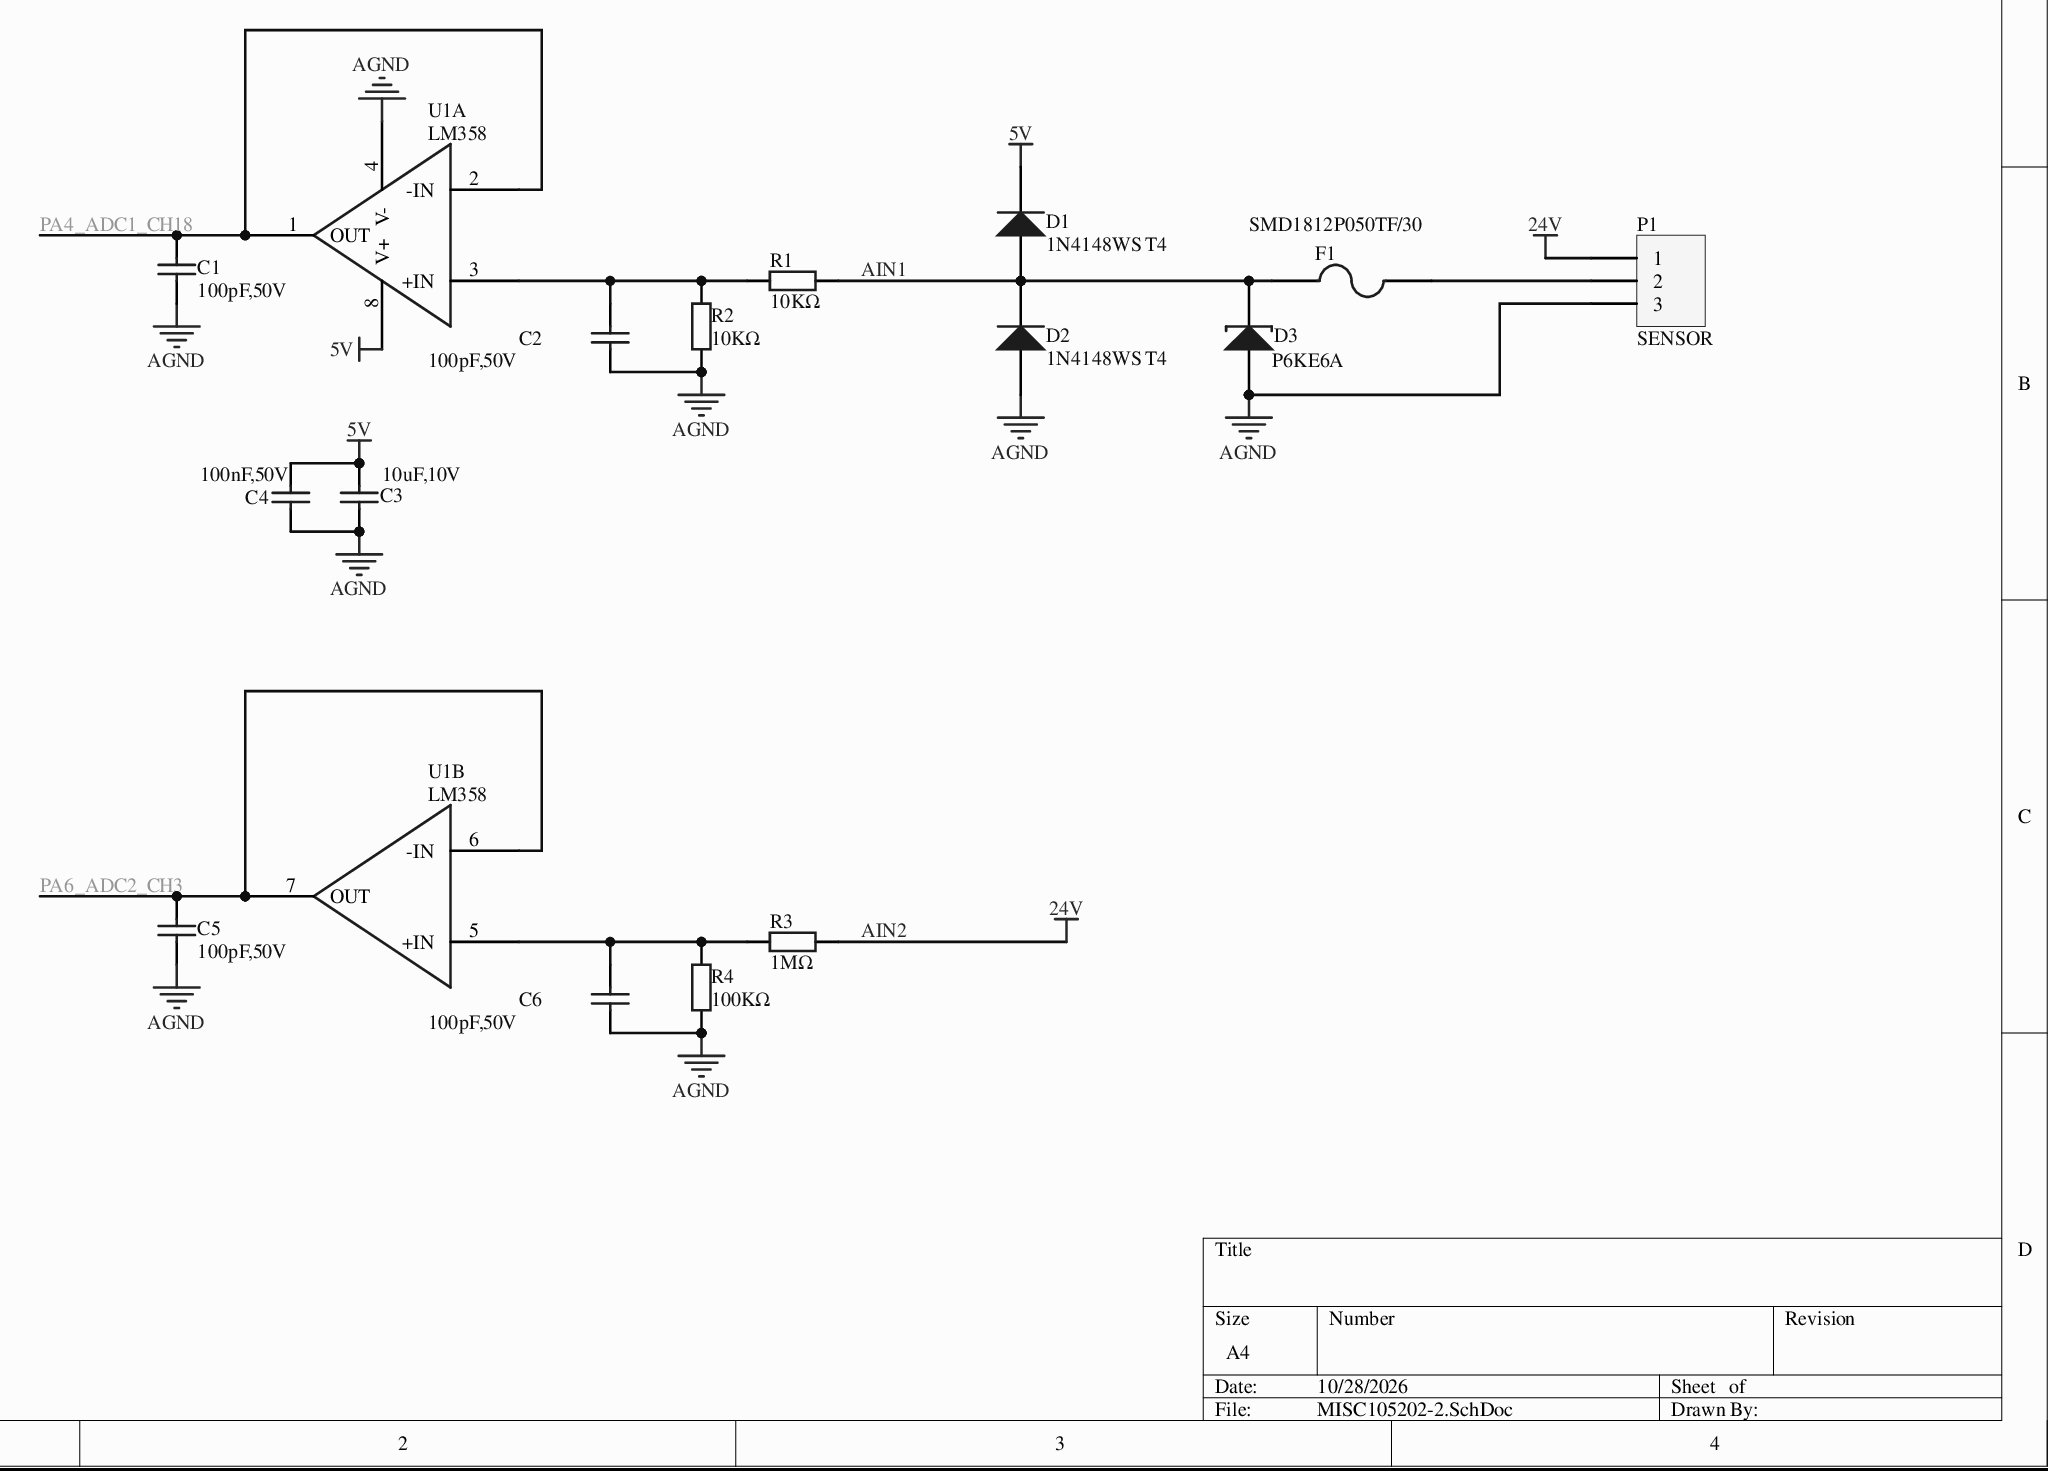
[diagram p0: MISC105202-2.SchDoc]
# Altium project MISC105202-19.PrjPCB (part 1 of 3)
7 sheets, 181 parts. Net scope: global (net labels, ports and power ports of the same name join across sheets).
Board file: MISC105202-15.PcbDoc
Sheets:
  MISC105202-2.SchDoc
  MISC105202-4.SchDoc
  PCBE105202.SchDoc
  MISC105202-9.SchDoc
  MISC105202-21.SchDoc
  MISC105202-13.SchDoc
  MISC105202-24.SchDoc

## Sheet MISC105202-2.SchDoc
size A4

### Parts
C1  100pF,50V  [0603_C]
C2  100pF,50V  [0603_C]
C3  10uF,10V  [0603_C]
C4  100nF,50V  [0603_C]
C5  100pF,50V  [0603_C]
C6  100pF,50V  [0603_C]
D1  1N4148WS T4  [SOD-323]
D2  1N4148WS T4  [SOD-323]
D3  P6KE6A  [P6KESMD]
F1  SMD1812P050TF/30  [1812]
P1  SENSOR  [508*3]
R1  10KΩ  [0603_R]
R2  10KΩ  [0603_R]
R3  1MΩ  [0603_R]
R4  100KΩ  [0603_R]
U1  LM358  [SO-8]  (parts A,B of 2)

### Nets
5V: C3.2 C4.2 D1.2(K) U1.8(V+)
AGND: C1.1 C2.1 C3.1 C4.1 C5.1 C6.1 D2.1(A) D3.1(A) P1.3 R2.1 R4.1 U1.4(V-)
AIN2: P1.1 R3.2  [also labelled 24V]
AIN1: D1.1(A) D2.2(K) D3.2(K) F1.2 R1.2
PA4_ADC1_CH18: C1.2 U1.1(OUT) U1.2(-IN)
PA6_ADC2_CH3: C5.2 U1.6(-IN) U1.7(OUT)
NetC2_2: C2.2 R1.1 R2.2 U1.3(+IN)
NetC6_2: C6.2 R3.1 R4.2 U1.5(+IN)
NetF1_1: F1.1 P1.2

### Library data of the parts
C1 C2 C5 C6 = 0603 100pF (101) 5% 50V: 贴片电容; ComponentLink1Description: supplier link; Package: 0603; Supplier: LC; SuppliersPartNumber: C14858
C3 = 0603 10uF (106) 10% 10V: 贴片电容; ComponentLink1Description: supplier link; Package: 0603; Supplier: LC; SuppliersPartNumber: C19702
C4 = 0603 100nF (104) 10% 50V: 贴片电容; ComponentLink1Description: supplier link; Package: 0603; Supplier: LC; SuppliersPartNumber: C14663
D1 D2 = SOD-323 1N4148WS T4: 二极管; ComponentLink1Description: supplier link; Package: SOD-323; Supplier: LC; SuppliersPartNumber: C2128
D3 = D Tunnel2: Tunnel Diode - Dependent Source Model; Published: 15-Apr-2002; LatestRevisionDate: 17-Jul-2002; LatestRevisionNote: Re-released for DXP Platform.; PackageReference: DIODE-0.4; Publisher: Altium Limited
F1 = Fuse 2: Fuse; Published: 8-Jun-2000; LatestRevisionDate: 17-Jul-2002; LatestRevisionNote: Re-released for DXP Platform.; PackageReference: PIN-W2/E2.8; Publisher: Altium Limited
P1 = Header 3: Header, 3-Pin; LatestRevisionDate: 17-Jul-2002; LatestRevisionNote: Re-released for DXP Platform.; Publisher: Altium Limited
R1-R4 = 0603 10KΩ (1002) 1%: 贴片电阻; ComponentLink1Description: supplier link; Package: 0603; Supplier: LC; SuppliersPartNumber: C25804
U1 = OPA2335

## Sheet MISC105202-4.SchDoc
size A4
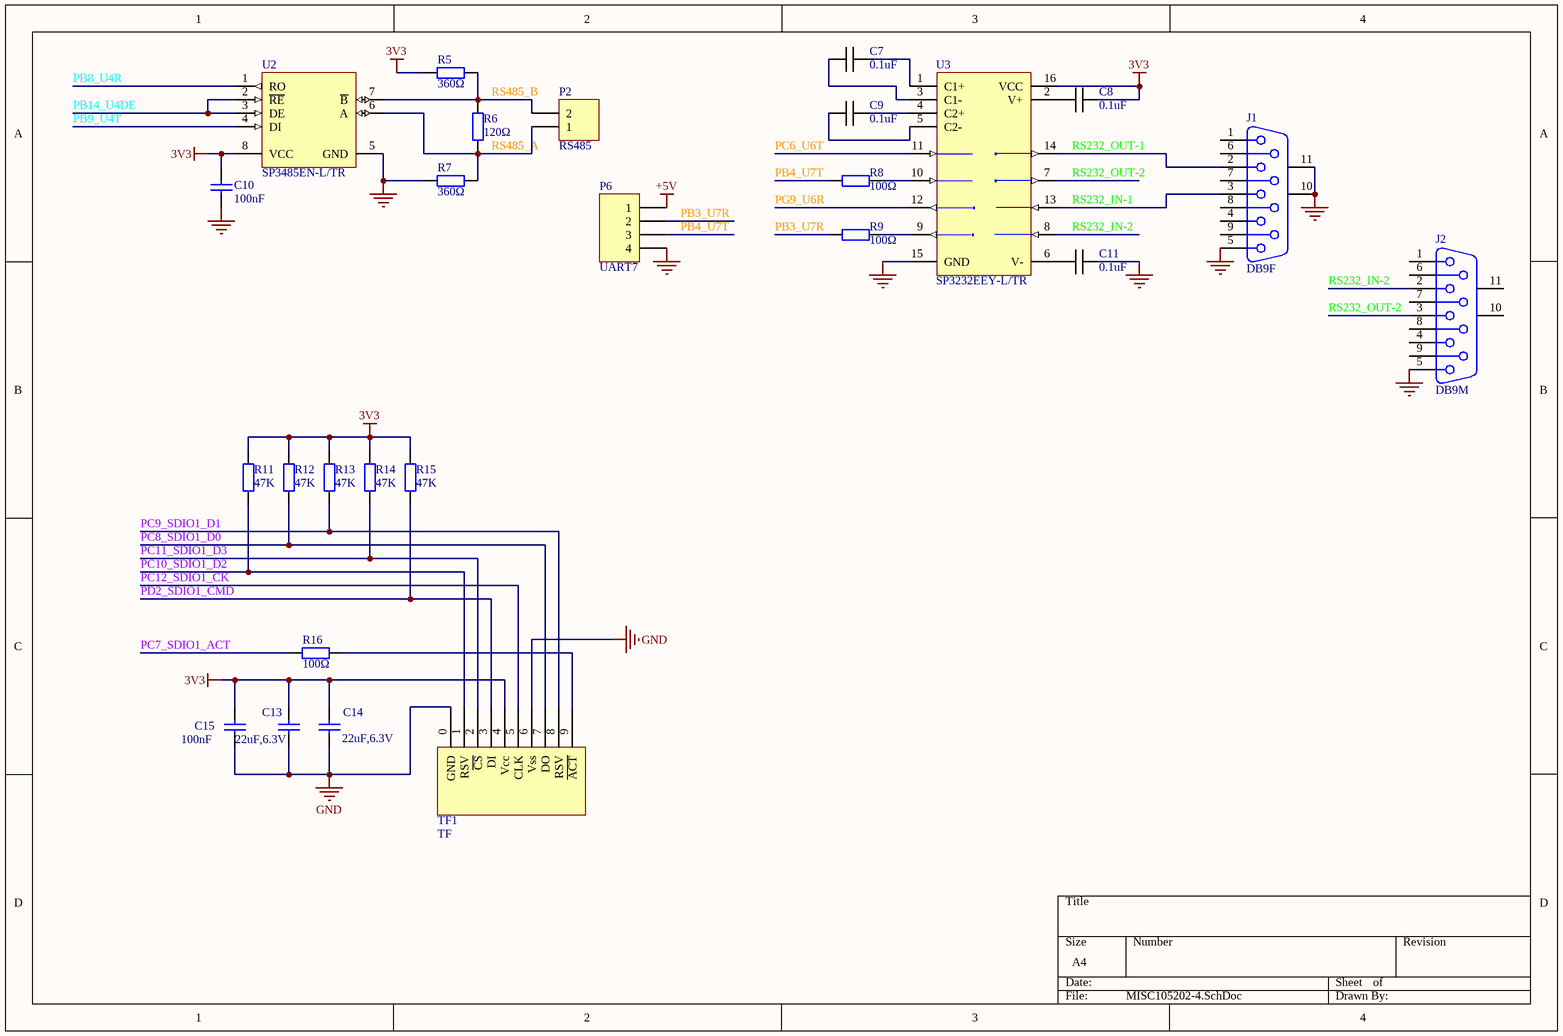
[diagram p1: MISC105202-4.SchDoc]

### Parts
C7  0.1uF  [0603_C]
C8  0.1uF  [0603_C]
C9  0.1uF  [0603_C]
C10  100nF  [0603_C]
C11  0.1uF  [0603_C]
C13  22uF,6.3V  [0603_C]
C14  22uF,6.3V  [0603_C]
C15  100nF  [0402_C]
J1  DB9F  [DB9RA/F]
J2  DB9M  [DB9RA/M]
P2  RS485  [508*2B]
P6  UART7  [HDR1X4]
R5  360Ω  [0603_R]
R6  120Ω  [0603_R]
R7  360Ω  [0603_R]
R8  100Ω  [0603_R]
R9  100Ω  [0603_R]
R11  47K  [0402_R]
R12  47K  [0402_R]
R13  47K  [0402_R]
R14  47K  [0402_R]
R15  47K  [0402_R]
R16  100Ω  [0402_R]
TF1  TF  [MICROSD]
U2  SP3485EN-L/TR  [SOIC-8_150mil]
U3  SP3232EEY-L/TR  [TSSOP-16]

### Nets
3V3: C8.1 C10.2 C13.2 C14.2 C15.2 R5.1 R11.2 R12.2 R13.2 R14.2 R15.2 TF1.4(Vcc) U2.8(VCC) U3.16(VCC)
+5V: P6.1
GND: C10.1 C11.1 C13.1 C14.1 C15.1 J1.5 J1.10(MH1) J1.11(MH2) J2.5 P6.4 R7.1 TF1.0(GND) TF1.6(Vss) U2.5(GND) U3.15(GND)
PB3_U7R: P6.2 R9.1  [project net PB3_SDIO2_D2]
PB4_U7T: P6.3 R8.1  [project net PB4_SDIO2_D3]
PB8_U4R: U2.1(RO)  [project net PB8_SDIO1_CKIN]
PB9_U4T: U2.4(DI)  [project net PB9_SDIO1_CDIR]
PB14_U4DE: U2.2(~{RE}) U2.3(DE)  [project net PB14_SDIO2_D0]
PC6_U6T: U3.11(T1IN)  [project net PC6_SDIO1_D0DIR]
PC7_SDIO1_ACT: R16.1
PC8_SDIO1_D0: R12.1 TF1.7(DO)
PC9_SDIO1_D1: R13.1 TF1.8(RSV)
PC10_SDIO1_D2: R11.1 TF1.1(RSV)
PC11_SDIO1_D3: R14.1 TF1.2(~{CS})
PC12_SDIO1_CK: TF1.5(CLK)
PD2_SDIO1_CMD: R15.1 TF1.3(DI)
PG9_U6R: U3.12(R1OUT)  [project net PG9_QSPI_BK2_IO2]
RS232_IN-1: J1.3 U3.13(R1IN)
RS232_IN-2: J2.2 U3.8(R2IN)
RS232_OUT-1: J1.2 U3.14(T1OUT)
RS232_OUT-2: J2.3 U3.7(T2OUT)
RS485_A: P2.1 R6.2 R7.2 U2.6(A)
RS485_B: P2.2 R5.2 R6.1 U2.7(~{B})
NetC7_1: C7.1 U3.1(C1+)
NetC7_2: C7.2 U3.3(C1-)
NetC8_2: C8.2 U3.2(V+)
NetC9_1: C9.1 U3.4(C2+)
NetC9_2: C9.2 U3.5(C2-)
NetC11_2: C11.2 U3.6(V-)
NetR8_2: R8.2 U3.10(T2IN)
NetR9_2: R9.2 U3.9(R2OUT)
NetR16_2: R16.2 TF1.9(~{ACT})

Not connected (* = marked no-connect by the designer): J1 1 4 6 7 8 9; J2 1 4 6 7 8 9 10(MH1) 11(MH2)

### Library data of the parts
C7-C9 C11 = CAP
C10 = 0603 100nF (104) 10% 50V: 贴片电容; ComponentLink1Description: supplier link; Package: 0603; Supplier: LC; SuppliersPartNumber: C14663
C13 C14 = 0603 22uF (226) 20% 6.3V: 贴片电容; ComponentLink1Description: supplier link; Package: 0603; Supplier: LC; SuppliersPartNumber: C59461
C15 = 0402 100nF (104) 10% 16V: 贴片电容; ComponentLink1Description: supplier link; Package: 0402; Supplier: LC; SuppliersPartNumber: C1525
J1 J2 = D Connector 9: Receptacle Assembly, 9 Position, Right Angle; PackageDocument: O; Positions: 9; Published: 15-Jun-2001; LatestRevisionDate: 17-Jul-2002; LatestRevisionNote: Re-released for DXP Platform.; DatasheetDocument: 1-Sep-1999; PackageReference: 788750; Orientation: Right Angle; Gender: Receptacle; Publisher: Altium Limited
P2 = Header 2: Header, 2-Pin; LatestRevisionDate: 17-Jul-2002; LatestRevisionNote: Re-released for DXP Platform.; Publisher: Altium Limited
P6 = Header 4: Header, 4-Pin; LatestRevisionDate: 17-Jul-2002; LatestRevisionNote: Re-released for DXP Platform.; Publisher: Altium Limited
R5 R7 = 0603 360Ω (3600) 1%: 贴片电阻; ComponentLink1Description: supplier link; Package: 0603; Supplier: LC; SuppliersPartNumber: C25194
R6 = 0603 120Ω (1200) 1%: 贴片电阻; ComponentLink1Description: supplier link; Package: 0603; Supplier: LC; SuppliersPartNumber: C22787
R8 R9 = 0603 100Ω (1000) 1%: 贴片电阻; ComponentLink1Description: supplier link; Package: 0603; Supplier: LC; SuppliersPartNumber: C22775
R11-R15 = 0402 47KΩ (4702) 1%: 贴片电阻; ComponentLink1Description: supplier link; Package: 0402; Supplier: LC; SuppliersPartNumber: C25792
R16 = 0402 100Ω (1000) 1%: 贴片电阻; ComponentLink1Description: supplier link; Package: 0402; Supplier: LC; SuppliersPartNumber: C25076
U2 = SP3485EN-L/TR_[C8963]: RS-485/RS-422; ComponentLink1Description: supplier link; Package: SOIC-8; Supplier: LC; SuppliersPartNumber: C8963
U3 = SP3232EEY-L/TR: RS232; ComponentLink1Description: supplier link; Package: TSSOP-16; Supplier: LC; SuppliersPartNumber: C13482

## Sheet PCBE105202.SchDoc
size A3; SheetNumber: 12; SheetTotal: 14
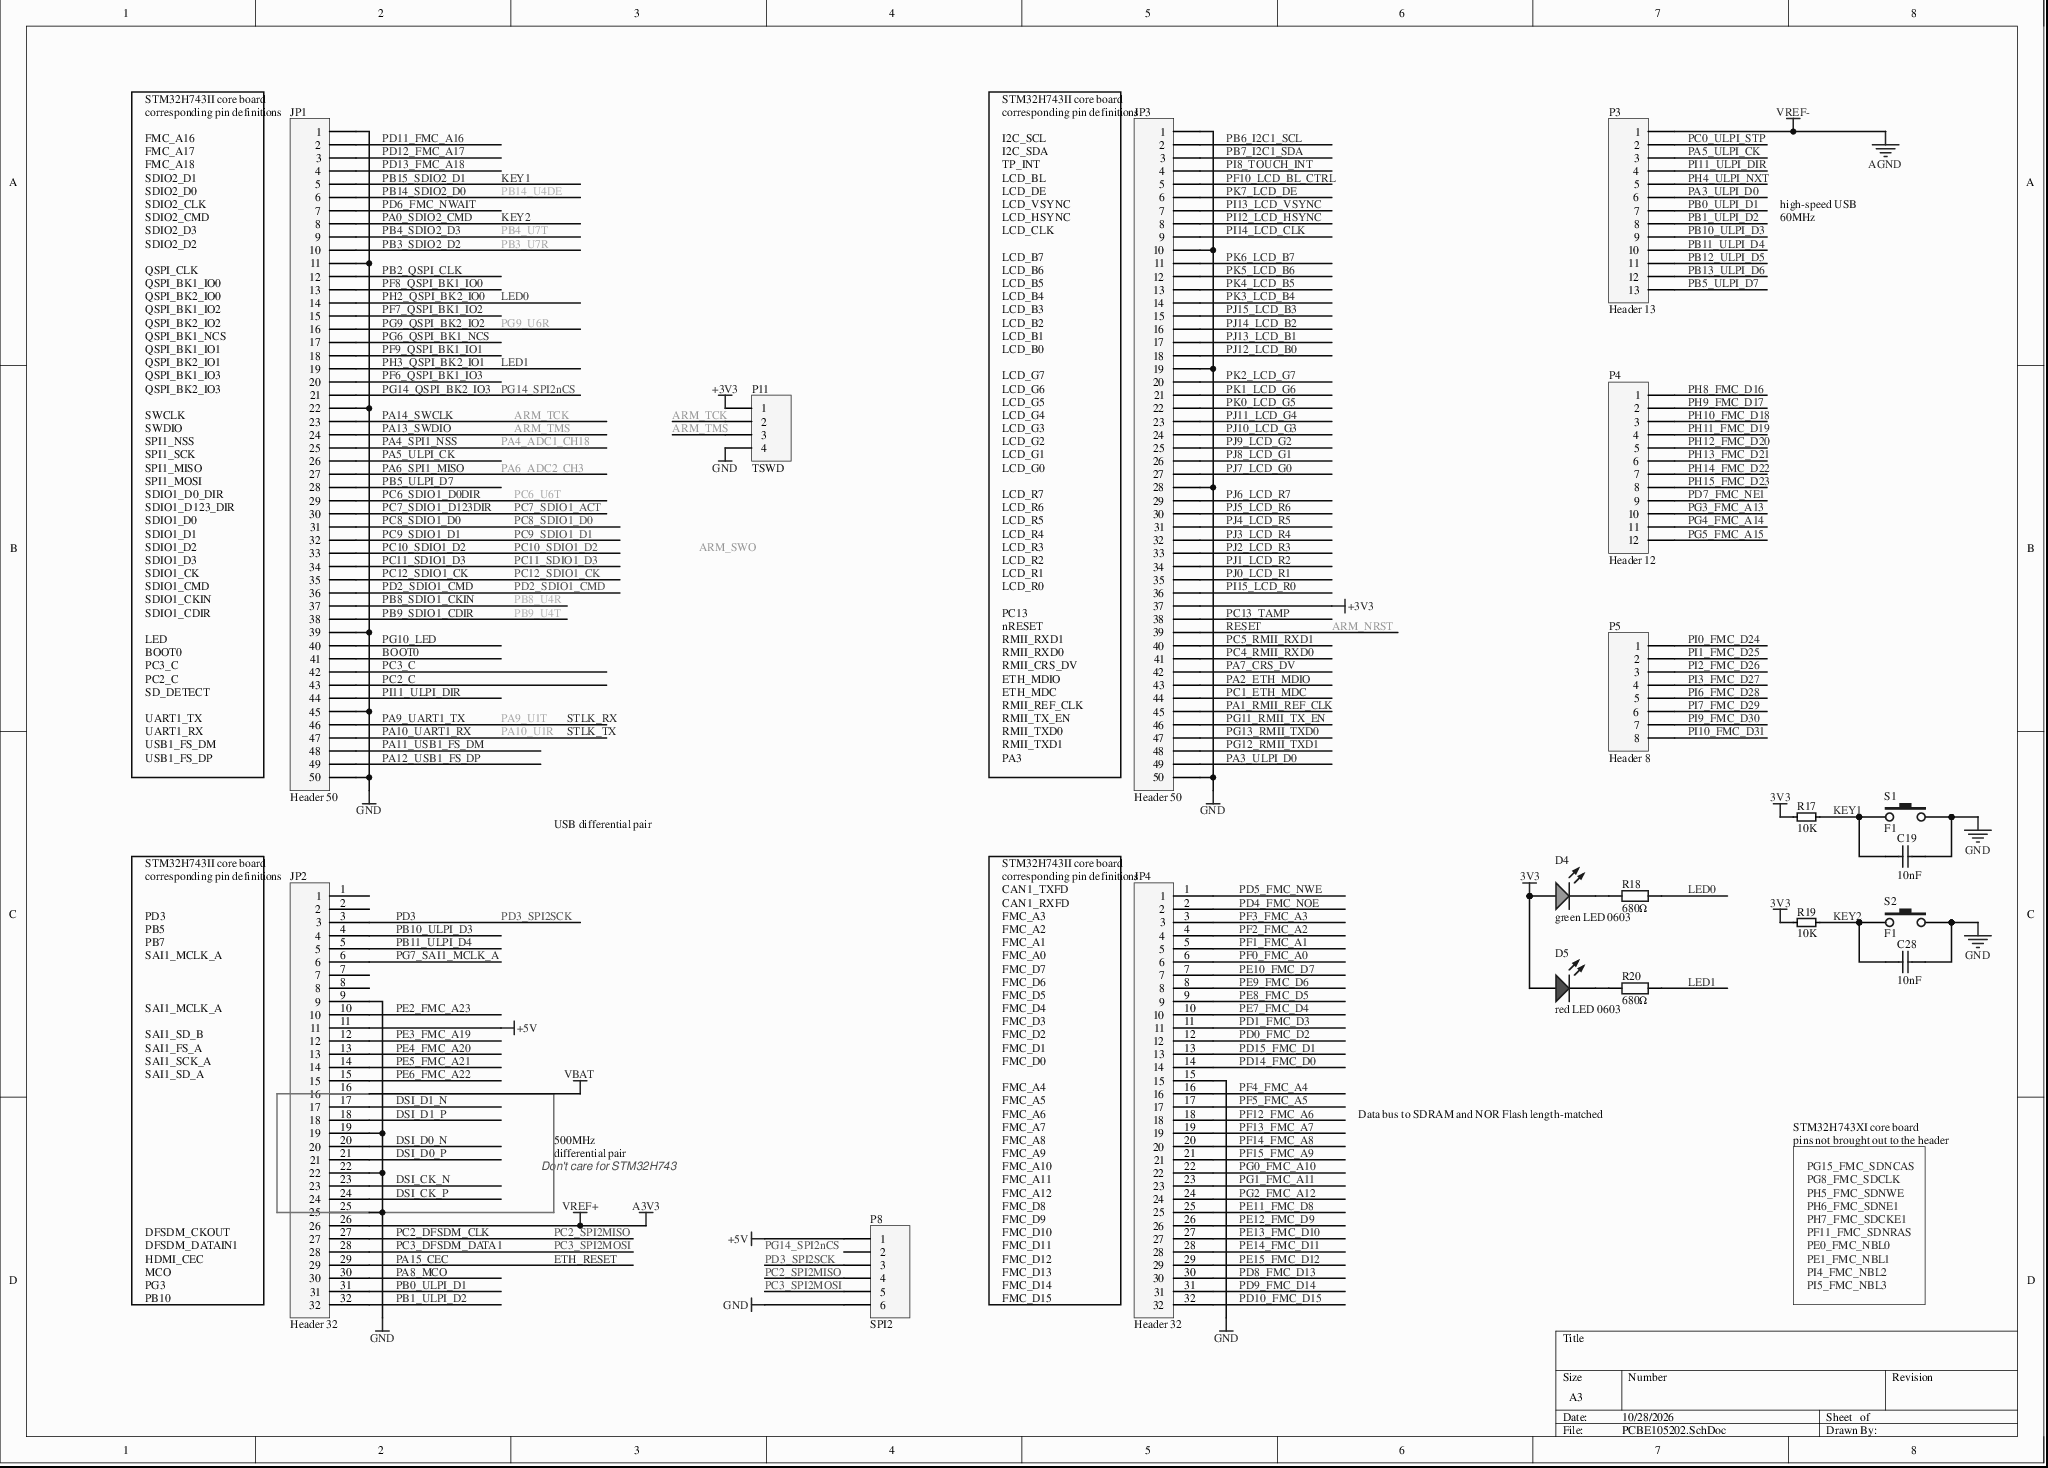
[diagram p2: PCBE105202.SchDoc]

### Parts
C19  10nF  [0603_C]
C28  10nF  [0603_C]
D4  green LED 0603  [0603_LED_S1]
D5  red LED 0603  [0603_LED_S1]
JP1  Header 50  [SIP-50-1.27-SMD-R]
JP2  Header 32  [SIP-32-1.27-SMD-R]
JP3  Header 50  [SIP-50-1.27-SMD]
JP4  Header 32  [SIP-32-1.27-SMD]
P3  Header 13  [CN13SM]
P4  Header 12  [CN12SM]
P5  Header 8  [CN8SM]
P8  SPI2  [HDR1X6]
P11  TSWD  [HDR1X4]
R17  10K  [0603_R]
R18  680Ω  [0603_R]
R19  10K  [0603_R]
R20  680Ω  [0603_R]
S1  F1  [Reset_TE]
S2  F1  [Reset_TE]

### Blocks framed on the sheet
Don't care for STM32H743: JP2

### Nets
3V3: D4.A D5.A R17.2 R19.2
+3V3: JP3.37 P11.1
+5V: JP2.11 P8.1
A3V3: JP2.26  [also labelled VREF+]
AGND: P3.1  [also labelled VREF-]
GND: C19.2 C28.2 JP1.1 JP1.11 JP1.22 JP1.39 JP1.45 JP1.50 JP2.9 JP2.19 JP2.22 JP2.25 JP3.1 JP3.10 JP3.19 JP3.28 JP3.50 JP4.15 P8.6 P11.4 S1.2 S2.2
VBAT: JP2.16
ARM_NRST: JP3.39  [also labelled ~{RESET}]
ARM_TCK: JP1.23 P11.2  [also labelled PA14_SWCLK]
ARM_TMS: JP1.24 P11.3  [also labelled PA13_SWDIO]
BOOT0: JP1.41
DSI_CK_N: JP2.23
DSI_CK_P: JP2.24
DSI_D0_N: JP2.20
DSI_D0_P: JP2.21
DSI_D1_N: JP2.17
DSI_D1_P: JP2.18
ETH_RESET: JP2.29  [also labelled PA15_CEC]
KEY1: C19.1 JP1.5 R17.1 S1.1  [also labelled PB15_SDIO2_D1]
KEY2: C28.1 JP1.8 R19.1 S2.1  [also labelled PA0_SDIO2_CMD]
LED0: JP1.14 R18.2  [also labelled PH2_QSPI_BK2_IO0]
LED1: JP1.19 R20.2  [also labelled PH3_QSPI_BK2_IO1]
PA1_RMII_REF_CLK: JP3.45
PA2_ETH_MDIO: JP3.43
PA3_ULPI_D0: JP3.49 P3.6
PA4_ADC1_CH18: JP1.25  [also labelled PA4_SPI1_NSS]
PA5_ULPI_CK: JP1.26 P3.3
PA6_ADC2_CH3: JP1.27  [also labelled PA6_SPI1_MISO]
PA7_CRS_DV: JP3.42
PA8_MCO: JP2.30
PA9_U1T: JP1.46  [also labelled PA9_UART1_TX, STLK_RX]
PA10_U1R: JP1.47  [also labelled PA10_UART1_RX, STLK_TX]
PA11_USB1_FS_DM: JP1.48
PA12_USB1_FS_DP: JP1.49
PB0_ULPI_D1: JP2.31 P3.7
PB1_ULPI_D2: JP2.32 P3.8
PB2_QSPI_CLK: JP1.12
PB3_SDIO2_D2: JP1.10  [also labelled PB3_U7R]
PB4_SDIO2_D3: JP1.9  [also labelled PB4_U7T]
PB5_ULPI_D7: JP1.28 P3.13
PB6_I2C1_SCL: JP3.2
PB7_I2C1_SDA: JP3.3
PB8_SDIO1_CKIN: JP1.37  [also labelled PB8_U4R]
PB9_SDIO1_CDIR: JP1.38  [also labelled PB9_U4T]
PB10_ULPI_D3: JP2.4 P3.9
PB11_ULPI_D4: JP2.5 P3.10
PB12_ULPI_D5: P3.11
PB13_ULPI_D6: P3.12
PB14_SDIO2_D0: JP1.6  [also labelled PB14_U4DE]
PC0_ULPI_STP: P3.2
PC1_ETH_MDC: JP3.44
PC2_C: JP1.43
PC2_DFSDM_CLK: JP2.27 P8.4  [also labelled PC2_SPI2MISO]
PC3_C: JP1.42
PC3_DFSDM_DATA1: JP2.28 P8.5  [also labelled PC3_SPI2MOSI]
PC4_RMII_RXD0: JP3.41
PC5_RMII_RXD1: JP3.40
PC6_SDIO1_D0DIR: JP1.29  [also labelled PC6_U6T]
PC7_SDIO1_ACT: JP1.30  [also labelled PC7_SDIO1_D123DIR]
PC8_SDIO1_D0: JP1.31
PC9_SDIO1_D1: JP1.32
PC10_SDIO1_D2: JP1.33
PC11_SDIO1_D3: JP1.34
PC12_SDIO1_CK: JP1.35
PC13_TAMP: JP3.38
PD0_FMC_D2: JP4.12
PD1_FMC_D3: JP4.11
PD2_SDIO1_CMD: JP1.36
PD3: JP2.3 P8.3  [also labelled PD3_SPI2SCK]
PD4_FMC_NOE: JP4.2
PD5_FMC_NWE: JP4.1
PD6_FMC_NWAIT: JP1.7
PD7_FMC_NE1: P4.9
PD8_FMC_D13: JP4.30
PD9_FMC_D14: JP4.31
PD10_FMC_D15: JP4.32
PD11_FMC_A16: JP1.2
PD12_FMC_A17: JP1.3
PD13_FMC_A18: JP1.4
PD14_FMC_D0: JP4.14
PD15_FMC_D1: JP4.13
PE2_FMC_A23: JP2.10
PE3_FMC_A19: JP2.12
PE4_FMC_A20: JP2.13
PE5_FMC_A21: JP2.14
PE6_FMC_A22: JP2.15
PE7_FMC_D4: JP4.10
PE8_FMC_D5: JP4.9
PE9_FMC_D6: JP4.8
PE10_FMC_D7: JP4.7
PE11_FMC_D8: JP4.25
PE12_FMC_D9: JP4.26
PE13_FMC_D10: JP4.27
PE14_FMC_D11: JP4.28
PE15_FMC_D12: JP4.29
PF0_FMC_A0: JP4.6
PF1_FMC_A1: JP4.5
PF2_FMC_A2: JP4.4
PF3_FMC_A3: JP4.3
PF4_FMC_A4: JP4.16
PF5_FMC_A5: JP4.17
PF6_QSPI_BK1_IO3: JP1.20
PF7_QSPI_BK1_IO2: JP1.15
PF8_QSPI_BK1_IO0: JP1.13
PF9_QSPI_BK1_IO1: JP1.18
PF10_LCD_BL_CTRL: JP3.5
PF12_FMC_A6: JP4.18
PF13_FMC_A7: JP4.19
PF14_FMC_A8: JP4.20
PF15_FMC_A9: JP4.21
PG0_FMC_A10: JP4.22
PG1_FMC_A11: JP4.23
PG2_FMC_A12: JP4.24
PG3_FMC_A13: P4.10
PG4_FMC_A14: P4.11
PG5_FMC_A15: P4.12
PG6_QSPI_BK1_NCS: JP1.17
PG7_SAI1_MCLK_A: JP2.6
PG9_QSPI_BK2_IO2: JP1.16  [also labelled PG9_U6R]
PG10_LED: JP1.40
PG11_RMII_TX_EN: JP3.46
PG12_RMII_TXD1: JP3.48
PG13_RMII_TXD0: JP3.47
PG14_QSPI_BK2_IO3: JP1.21  [also labelled PG14_SPI2nCS]
PH4_ULPI_NXT: P3.5
PH8_FMC_D16: P4.1
PH9_FMC_D17: P4.2
PH10_FMC_D18: P4.3
PH11_FMC_D19: P4.4
PH12_FMC_D20: P4.5
PH13_FMC_D21: P4.6
PH14_FMC_D22: P4.7
PH15_FMC_D23: P4.8
PI0_FMC_D24: P5.1
PI1_FMC_D25: P5.2
PI2_FMC_D26: P5.3
PI3_FMC_D27: P5.4
PI6_FMC_D28: P5.5
PI7_FMC_D29: P5.6
PI8_TOUCH_INT: JP3.4
PI9_FMC_D30: P5.7
PI10_FMC_D31: P5.8
PI11_ULPI_DIR: JP1.44 P3.4
PI12_LCD_HSYNC: JP3.8
PI13_LCD_VSYNC: JP3.7
PI14_LCD_CLK: JP3.9
PI15_LCD_R0: JP3.36
PJ0_LCD_R1: JP3.35
PJ1_LCD_R2: JP3.34
PJ2_LCD_R3: JP3.33
PJ3_LCD_R4: JP3.32
PJ4_LCD_R5: JP3.31
PJ5_LCD_R6: JP3.30
PJ6_LCD_R7: JP3.29
PJ7_LCD_G0: JP3.27
PJ8_LCD_G1: JP3.26
PJ9_LCD_G2: JP3.25
PJ10_LCD_G3: JP3.24
PJ11_LCD_G4: JP3.23
PJ12_LCD_B0: JP3.18
PJ13_LCD_B1: JP3.17
PJ14_LCD_B2: JP3.16
PJ15_LCD_B3: JP3.15
PK0_LCD_G5: JP3.22
PK1_LCD_G6: JP3.21
PK2_LCD_G7: JP3.20
PK3_LCD_B4: JP3.14
PK4_LCD_B5: JP3.13
PK5_LCD_B6: JP3.12
PK6_LCD_B7: JP3.11
PK7_LCD_DE: JP3.6
NetD4_K: D4.K R18.1
NetD5_K: D5.K R20.1

Not connected (* = marked no-connect by the designer): JP2 1* 2* 7* 8*; P8 2

### Notes on the sheet
- STM32H743II core board
- (near JP3) STM32H743II core board
- FMC_A16
- FMC_A17
- FMC_A18
- (near JP1) corresponding pin definitions
- I2C_SCL
- I2C_SDA
- TP_INT
- (near JP3) corresponding pin definitions
- SDIO2_D0
- SDIO2_D1
- SDIO2_D3
- SDIO2_CLK
- SDIO2_CMD
- LCD_BL
- LCD_DE
- LCD_VSYNC
- LCD_HSYNC
- LCD_CLK
- 60MHz
- high-speed USB
- SDIO2_D2
- QSPI_BK1_IO0
- QSPI_BK2_IO0
- QSPI_CLK
- LCD_B7
- LCD_B4
- LCD_B5
- LCD_B6
- QSPI_BK1_IO1
- QSPI_BK1_IO2
- QSPI_BK2_IO1
- QSPI_BK2_IO2
- QSPI_BK1_NCS
- LCD_B0
- LCD_B1
- LCD_B2
- LCD_B3
- QSPI_BK1_IO3
- QSPI_BK2_IO3
- SWCLK
- SWDIO
- LCD_G3
- LCD_G4
- LCD_G5
- LCD_G6
- LCD_G7
- SPI1_NSS
- SPI1_SCK
- SPI1_MISO
- SPI1_MOSI
- SDIO1_D0_DIR
- LCD_G0
- LCD_G1
- LCD_G2
- LCD_R7
- SDIO1_D123_DIR
- SDIO1_D0
- SDIO1_D1
- SDIO1_D2
- SDIO1_D3
- LCD_R2
- LCD_R3
- LCD_R4
- LCD_R5
- LCD_R6
- SDIO1_CK
- SDIO1_CMD
- SDIO1_CKIN
- SDIO1_CDIR
- LCD_R0
- LCD_R1
- PC13
- nRESET
- LED
- BOOT0
- PC3_C
- PC2_C
- SD_DETECT
- RMII_RXD0
- RMII_RXD1
- RMII_CRS_DV
- ETH_MDIO
- ETH_MDC
- UART1_TX
- UART1_RX
- USB1_FS_DM
- USB1_FS_DP
- RMII_REF_CLK
- RMII_TX_EN
- RMII_TXD0
- RMII_TXD1
- PA3
- USB differential pair
- (near JP2) corresponding pin definitions
- CAN1_TXFD
- (near JP4) STM32H743II core board
- (near JP4) corresponding pin definitions
- PD3
- PB5
- PB7
- SAI1_MCLK_A
- CAN1_RXFD
- FMC_A0
- FMC_A1
- FMC_A2
- FMC_A3
- FMC_D3
- FMC_D4
- FMC_D5
- FMC_D6
- FMC_D7
- SAI1_SD_B
- SAI1_FS_A
- SAI1_SCK_A
- SAI1_SD_A
- FMC_A4
- FMC_D0
- FMC_D1
- FMC_D2
- 500MHz
- differential pair
- FMC_A5
- FMC_A6
- FMC_A7
- FMC_A8
- FMC_A9
- Data bus to SDRAM and NOR Flash length-matched
- STM32H743XI core board
- pins not brought out to the header
- FMC_A10
- FMC_A11
- FMC_A12
- FMC_D8
- FMC_D9
- DFSDM_CKOUT
- DFSDM_DATAIN1
- HDMI_CEC
- MCO
- PG3
- FMC_D10
- FMC_D11
- FMC_D12
- FMC_D13
- FMC_D14
- PB10
- FMC_D15
- Labels drawn without touching a wire or pin: ARM_SWO, PE0_FMC_NBL0, PE1_FMC_NBL1, PF11_FMC_SDNRAS, PG8_FMC_SDCLK, PG14_SPI2nCS, PG15_FMC_SDNCAS, PH5_FMC_SDNWE, PH6_FMC_SDNE1, PH7_FMC_SDCKE1, PI4_FMC_NBL2, PI5_FMC_NBL3

### Library data of the parts
C19 C28 = 0402 10nF (103) 10% 50V: 贴片电容; ComponentLink1Description: supplier link; Package: 0402; Supplier: LC; SuppliersPartNumber: C15195
D4 = 0603 绿灯: 发光二极管; ComponentLink1Description: supplier link; Package: 0603; Supplier: LC; SuppliersPartNumber: C72043
D5 = 0603 红灯: 发光二极管; ComponentLink1Description: supplier link; Package: 0603; Supplier: LC; SuppliersPartNumber: C2286
JP1 JP3 = Header 50: Header, 50-Pin; LatestRevisionDate: 17-Jul-2002; LatestRevisionNote: Re-released for DXP Platform.; Publisher: Altium Limited
P3 = Header 13: Header, 13-Pin; LatestRevisionDate: 17-Jul-2002; LatestRevisionNote: Re-released for DXP Platform.; Publisher: Altium Limited
P4 = Header 12: Header, 12-Pin; LatestRevisionDate: 17-Jul-2002; LatestRevisionNote: Re-released for DXP Platform.; Publisher: Altium Limited
P5 = Header 8: Header, 8-Pin; LatestRevisionDate: 17-Jul-2002; LatestRevisionNote: Re-released for DXP Platform.; Publisher: Altium Limited
P8 = Header 6: Header, 6-Pin; LatestRevisionDate: 17-Jul-2002; LatestRevisionNote: Re-released for DXP Platform.; Publisher: Altium Limited
P11 = Header 4: Header, 4-Pin; LatestRevisionDate: 17-Jul-2002; LatestRevisionNote: Re-released for DXP Platform.; Publisher: Altium Limited
R17 R19 = Reszte: Resistor
R18 R20 = 0603 680Ω (6800) 1%: 贴片电阻; ComponentLink1Description: supplier link; Package: 0603; Supplier: LC; SuppliersPartNumber: C23228
S1 S2 = SW-PB